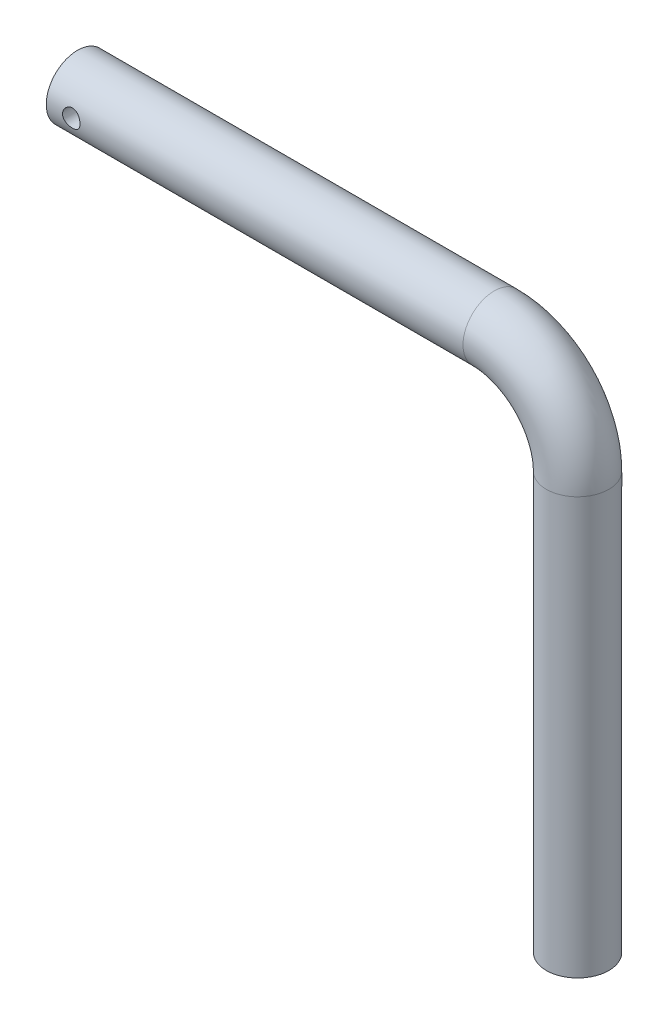
from build123d import *

# Parameters (mm, degrees)
SWEEP_1_PROFILE_R   = 7.5
SKETCH_6_R          = 2.1
CUT_EXTRUDE_1_DEPTH = 20


with BuildPart() as part:
    # 扫描1: sweep along a path in 草图1
    with BuildLine(Plane.XY) as sweep_1_path:
        Line((0, 0), (100, 0))
        ThreePointArc((100, 0), (114.142135624, -5.857864376), (120, -20))
        Line((120, -20), (120, -120))
    # 扫描1 profile (on start of the path) → 扫描1 (sweep)
    with BuildSketch(Plane(origin=(0, 0, 0), x_dir=(0, 0, 1), z_dir=(1, 0, 0))):
        Circle(SWEEP_1_PROFILE_R)
    sweep(path=sweep_1_path.line)

    # 草图6 → 切除-拉伸1 (cut)
    with BuildSketch(Plane.XY.offset(7.5)):
        with Locations((6, 0)):
            Circle(SKETCH_6_R)
    extrude(amount=-CUT_EXTRUDE_1_DEPTH, mode=Mode.SUBTRACT)


solid = part.part
